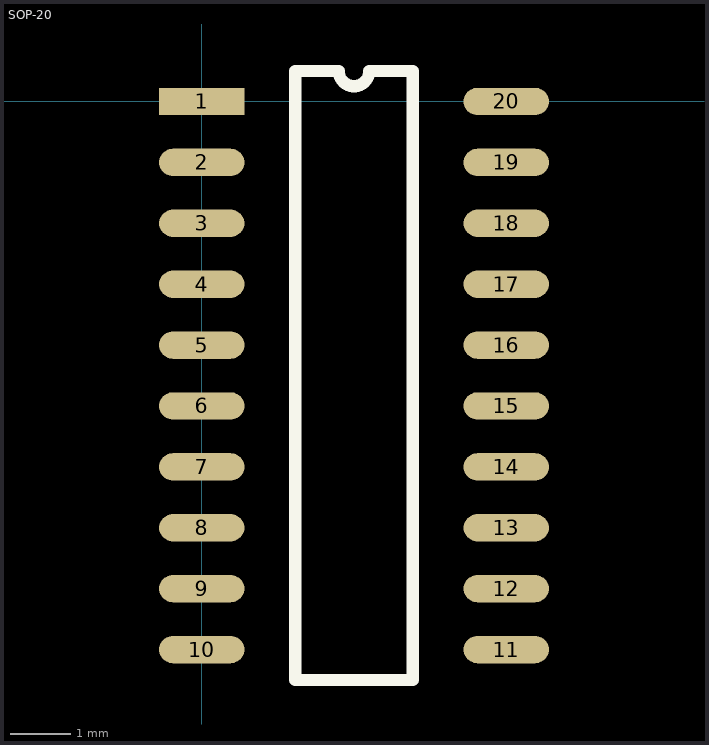
[diagram p0: the footprint, top view; thin cyan lines are the x and y axes]
# Altium footprint library MISC84379-2.PcbLib: 1 footprints
Each footprint in its own frame and in the unit in brackets; x right, y up, seen from the top. Pads: shape width x height; smd on the part's side, far side on the other; paste and mask are expansions set on the pad; w line width, h text height; cw(c..) or ccw(c..) is an arc to the next point about the centre after c.

## SOP-20 [mm]
pads (20):
  rect 1.4x0.45 smd: 1(0,0)
  oval 1.4x0.45 smd: 2(0,-1) 3(0,-2) 4(0,-3) 5(0,-4) 6(0,-5) 7(0,-6) 8(0,-7) 9(0,-8) 10(0,-9) 11(5,-9) 12(5,-8) 13(5,-7) 14(5,-6) 15(5,-5) 16(5,-4) 17(5,-3) 18(5,-2) 19(5,-1) 20(5,0)
Top Overlay:
  lines w0.2: 1.535,-9.5 3.465,-9.5 3.465,0.5 2.75,0.5 cw(c2.5,0.5) 2.25,0.5 1.535,0.5 1.535,-9.5